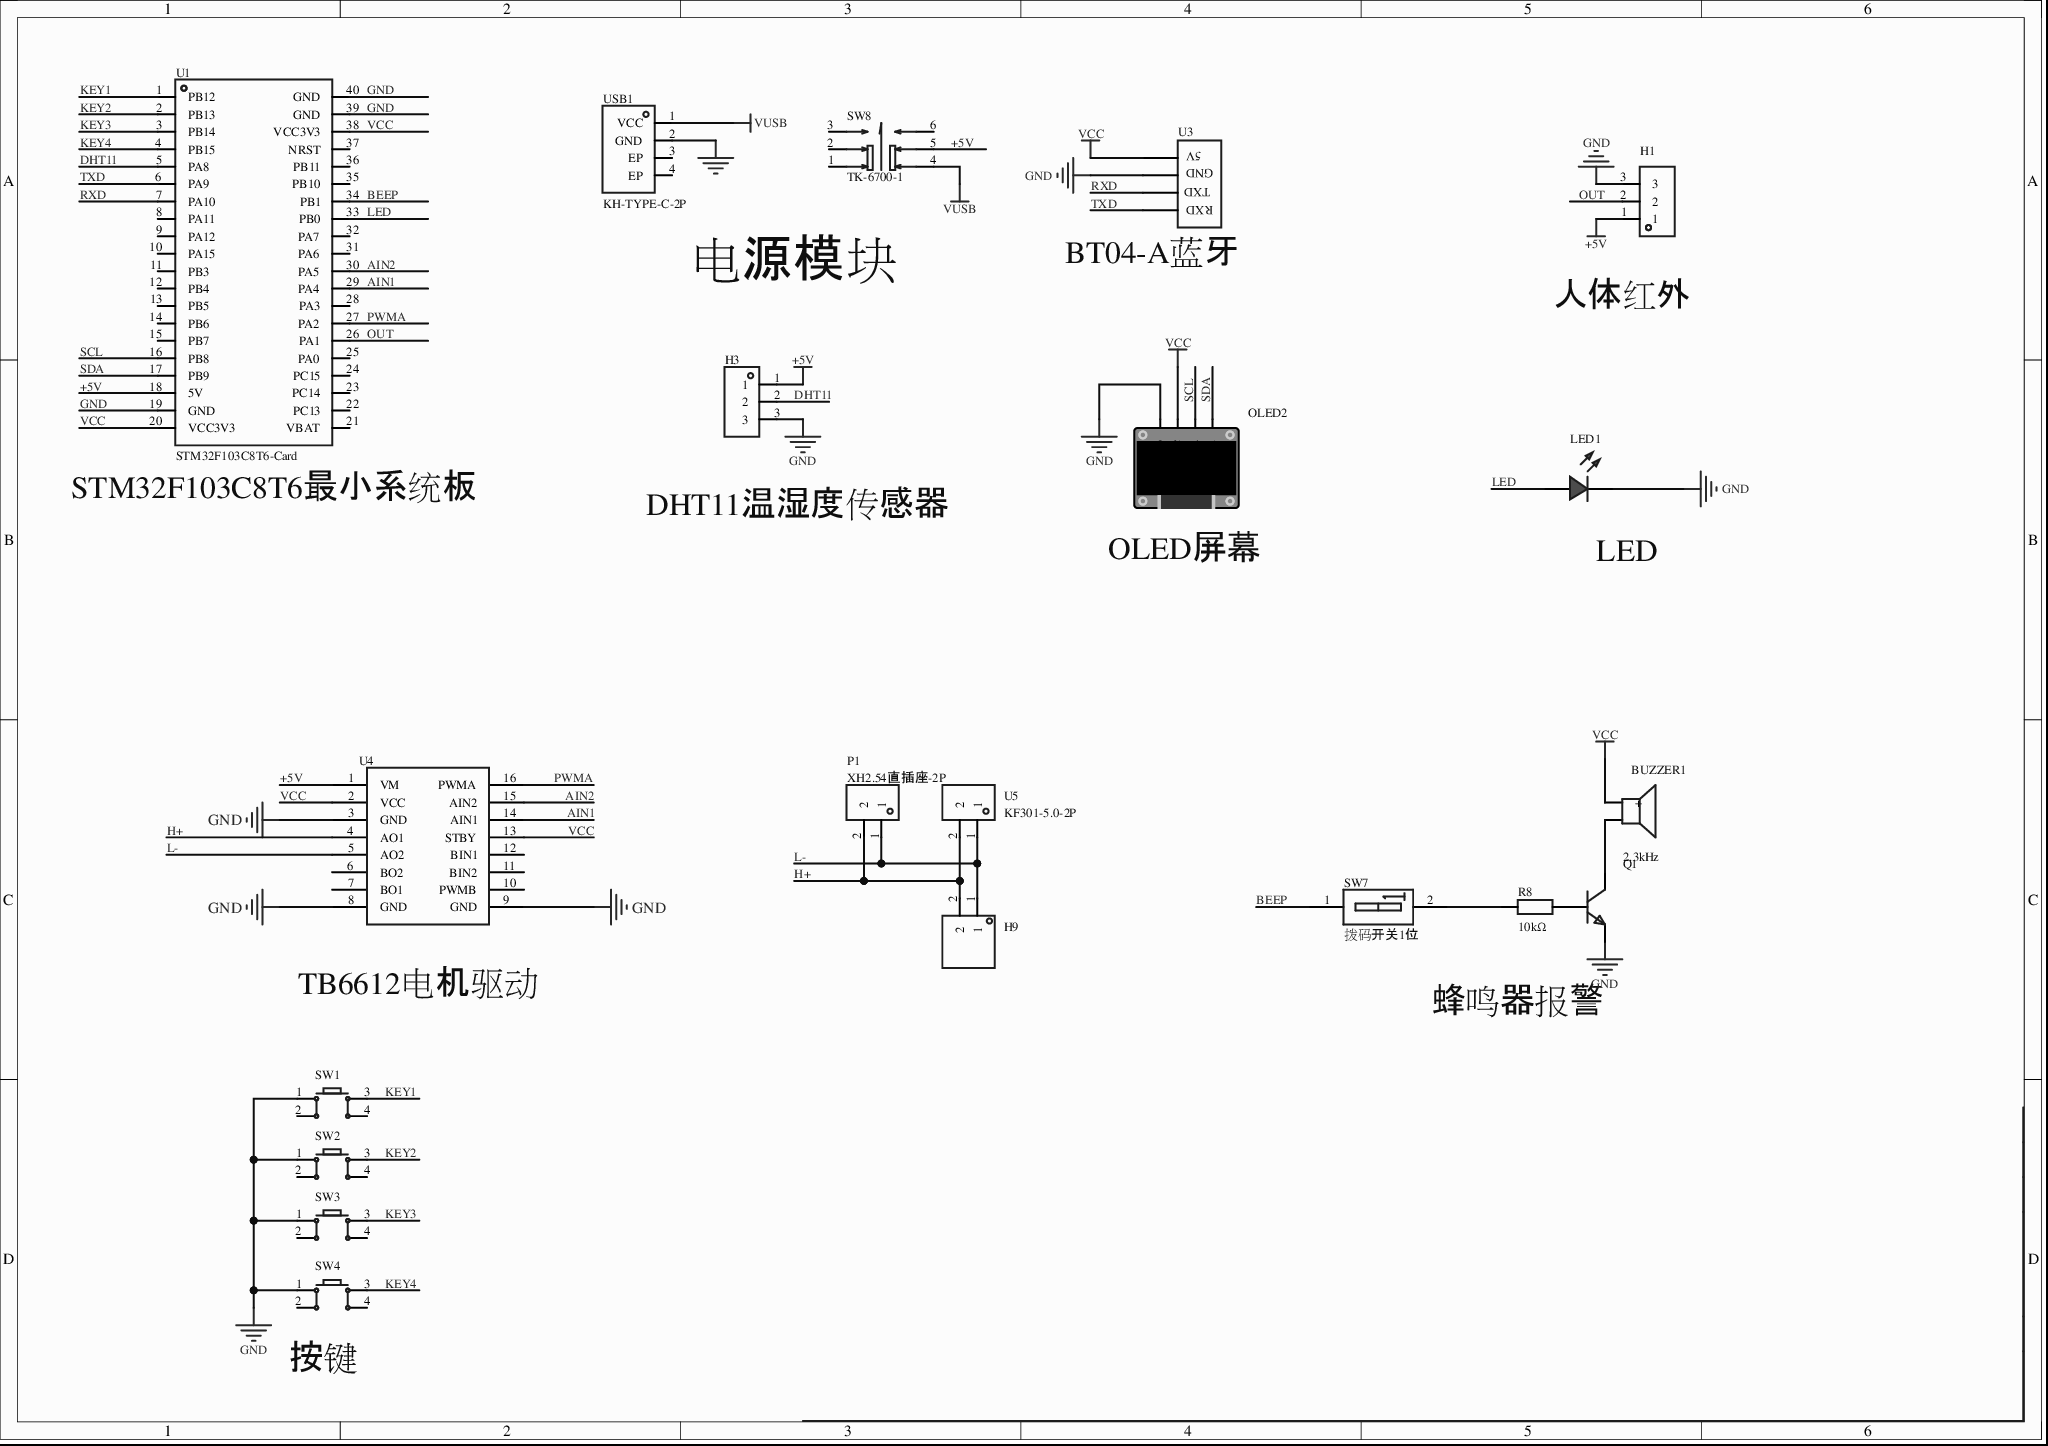
[diagram p0: MISC51405-3.schdoc]
# Altium project MISC51405-2.PrjPcb
1 sheet, 20 parts. Net scope: global (net labels, ports and power ports of the same name join across sheets).
Board file: MISC51405.pcbdoc

## Sheet MISC51405-3.schdoc
size 297 x 209 mm; Version: V1.0; @Project Name: MISC51405; @Page Count: 1; @Update Date: 2026-05-25; @Create Date: 2026-05-25; @Schematic Name: MISC51405; @Page No: 1; @Create Time: 23:22:16; @Update Time: 17:32:40; @Board Name: MISC51405

### Parts
BUZZER1  2.3kHz  [BUZ-TH_BD12.0-P7.60-D0.6-FD]
H1  (no value)  [HDR-TH_3P-P2.54-V-F]
H3  (no value)  [HDR-TH_3P-P2.54-V-F]
H9  (no value)  [HDR-TH_2P-P2.54-V-M-1]
LED1  (no value)  [LED_TH-3mm]
OLED2  (no value)  [0.96OLED_4P]
P1  XH2.54直插座-2P  [CONN-TH_XH2.54-2P]
Q1  (no value)  [S8050_TO_92]
R8  10kΩ  [Res_1/4W]
SW1  (no value)  [SW-TH_4P-L6.0-W6.0-P4.50-LS6.5]
SW2  (no value)  [SW-TH_4P-L6.0-W6.0-P4.50-LS6.5]
SW3  (no value)  [SW-TH_4P-L6.0-W6.0-P4.50-LS6.5]
SW4  (no value)  [SW-TH_4P-L6.0-W6.0-P4.50-LS6.5]
SW7  拨码开关1位  [SW-TH_2P-L3.9-W9.9-P2.54-LS7.6]
SW8  TK-6700-1  [SW-TH_TK-6700-1]
U1  STM32F103C8T6-Card  [CONN-TH_L53.3-W22.9_STM32F103C8T6-CARD]
U3  (no value)  [BT04-A]
U4  (no value)  [tb6612]
U5  KF301-5.0-2P  [CONN-TH_P5.00_KF301-5.0-2P]
USB1  KH-TYPE-C-2P  [USB-SMD_KH-TYPE-C-2P]

### Nets
+5V: H1.1 H3.1 SW8.5 U1.18(5V) U4.1(VM)
GND: H1.3 H3.3 LED1.2(A) OLED2.1(GND) Q1.1(E) SW1.1 SW2.1 SW3.1 SW4.1 U1.19(GND) U1.39(GND) U1.40(GND) U3.3 U4.3(GND) U4.8(GND) U4.9(GND) USB1.2(GND)
VCC: BUZZER1.1(+) OLED2.2(VCC) U1.20(VCC3V3) U1.38(VCC3V3) U3.4 U4.2(VCC) U4.13(STBY)
VUSB: SW8.4 USB1.1(VCC)
AIN1: U1.29(PA4) U4.14(AIN1)
AIN2: U1.30(PA5) U4.15(AIN2)
BEEP: SW7.1(A1) U1.34(PB1)
DHT11: H3.2 U1.5(PA8)
H+: H9.2 P1.2 U4.4(AO1) U5.2
KEY1: SW1.3 U1.1(PB12)
KEY2: SW2.3 U1.2(PB13)
KEY3: SW3.3 U1.3(PB14)
KEY4: SW4.3 U1.4(PB15)
L-: H9.1 P1.1 U4.5(AO2) U5.1
LED: LED1.1(C) U1.33(PB0)
OUT: H1.2 U1.26(PA1)
PWMA: U1.27(PA2) U4.16(PWMA)
RXD: U1.7(PA10) U3.2
SCL: OLED2.3(SCL) U1.16(PB8)
SDA: OLED2.4(SDA) U1.17(PB9)
TXD: U1.6(PA9) U3.1
NetBUZZER1_2: BUZZER1.2 Q1.3(C)
NetQ1_2: Q1.2(B) R8.2
NetR8_1: R8.1 SW7.2(A2)

Not connected (* = marked no-connect by the designer): SW1 2 4; SW2 2 4; SW3 2 4; SW4 2 4; SW8 1* 2* 3* 6*; U1 8(PA11) 9(PA12) 10(PA15) 11(PB3) 12(PB4) 13(PB5) 14(PB6) 15(PB7) 21(VBAT) 22(PC13) 23(PC14) 24(PC15) 25(PA0) 28(PA3) 31(PA6) 32(PA7) 35(PB10) 36(PB11) 37(NRST); U4 6(BO2) 7(BO1) 10(PWMB) 11(BIN2) 12(BIN1); USB1 3(EP) 4(EP)

### Notes on the sheet
- 电源模块
- (near U3) BT04-A蓝牙
- (near H1) 人体红外
- (near U1) STM32F103C8T6最小系统板
- DHT11温湿度传感器
- OLED屏幕
- (near LED1) LED
- TB6612电机驱动
- 蜂鸣器报警
- (near SW4) 按键

### Library data of the parts
BUZZER1 = TMB12A05_C96093: 驱动方式:有源(内含驱动线路);构造类型:电磁式;额定电压:5V;频率:2.3kHz;声压(SPL):85dB@5V,10cm;; Manufacturer: 华能; 3D Model: 16ab50e14c5b4f2c986c135bdba60e37; 3D Model Transform: 472.44,472.176,0,90,0,0,-0.787,0,-177.165; Technology Type: 电磁式; Rated Voltage: 5V; Operating Voltage: 4V~8V; AddInBom: yes; ModelName: BUZ-TH_D12.0-H9.5-P7.60; Symbol: TMB12A05; Device: TMB12A05_C96093; LCSC Part Name: TMB12A05; Supplier Part: C96093; Manufacturer Part: TMB12A05; Supplier Footprint: 插件,D=12mm; JLCPCB Part Class: Extended Part; Datasheet: https://atta.szlcsc.com/upload/public/pdf/source/20170522/1495448324811.pdf; Supplier: LCSC; Oscillator Circuit: 有源(内含驱动线路); Value: 2.3kHz; Sound Pressure Level (SPL): 85dB@5V,10cm; Diameter (φD): 12mm; Height: 9.8mm; ConvertToPcb: yes; FootprintName: BUZ-TH_BD12.0-P7.60-D0.6-FD
H1 = HDR-F_2.54_1x3P: Symbol: PM254V-11-03-H85; ConvertToPcb: yes; ModelId: f3b3cc5aae9641bf9e56fc160cef875b; ModelName: HDR2.54-F-LI-1X3P; ModelTransform: 299.9994,100,0,0,0,0,0,0,-118.11; Device: HDR-F_2.54_1x3P; FootprintName: HDR-TH_3P-P2.54-V-F; AddInBom: yes; SupplierPart: C541850; Supplier Footprint: 插件
H3 = HDR-F_2.54_1x3P: Symbol: PM254V-11-03-H85; 3D Model: f3b3cc5aae9641bf9e56fc160cef875b; 3D Model Transform: 299.9994,100,0,0,0,0,0,0,-118.11; ConvertToPcb: yes; ModelName: HDR2.54-F-LI-1X3P; Device: HDR-F_2.54_1x3P; Supplier Part: C541850; Supplier Footprint: 插件; FootprintName: HDR-TH_3P-P2.54-V-F; AddInBom: yes
H9 = HDR-M_2.54_1x2P: Symbol: 210S-1*2P L=11.6MMGold-plated black; ConvertToPcb: yes; ModelId: 79b2e9f2d70a4d68a1b7098f27c6d4c50819f05c4eef4c71ace90d822a990e87; ModelName: HDR-M-2.54_1x2; ModelTransform: 200,100,0,0,0,0,0,0,-118.11; Device: HDR-M_2.54_1x2P; AddInBom: yes; SupplierPart: C124375; Supplier Footprint: 插件; FootprintName: HDR-TH_2P-P2.54-V-M-1
LED1 = LED_TH-R_3mm: ConvertToPcb: yes; ModelId: a497c992633541038a38947cdc58012f0819f05c4eef4c71ace90d822a990e87; ModelName: LED-TH-3mm_R; ModelTransform: 141.274,153.327,0,0,0,0,-5.984,0,-137.795; Symbol: LED_TH-R; Device: LED_TH-R_3mm; AddInBom: yes; FootprintName: LED_TH-3mm; Supplier Footprint: 插件
OLED2 = 0.96OLED模块_4P: ConvertToPcb: yes; ModelId: 79c000fdb68d45a296c2e9bedf4f9055; ModelTransform: 1393.69792,1318.895,0,0,0,0,0,-560.079,-137.795; Symbol: 0.96OLED模块_4P; Device: 0.96OLED模块_4P; AddInBom: yes; FootprintName: 0.96OLED_4P; Supplier Footprint: 插件; ModelName: 0.96OLED_4P
P1 = XH2.54直插座-2P: AddInBom: yes; ModelId: c3cc11bd8b8748c1ae6bc231aac3a1ff0819f05c4eef4c71ace90d822a990e87; ModelTransform: 296.889,230.315,0,0,0,0,0,26.653,-137.795; Symbol: XH2.54直插座-2P; Device: XH2.54直插座-2P; LCSC Part Name: XH2.54直插座-2P; SupplierPart: C9900016957; ManufacturerPart: XH2.54直插座-2P; Supplier Footprint: XH2.54-2; JLCPCB Part Class: Extended Part; Supplier: LCSC; ConvertToPcb: yes; FootprintName: CONN-TH_XH2.54-2P; ModelName: CONN-TH_XH2.54-2P
Q1 = S8050_TO_NPN: 3D Model: aafe8e06f2154e7c93506efd0d6632dd; 3D Model Transform: 180.78,141.44,417.3,0,0,0,0,0,-200; ConvertToPcb: yes; ModelName: TO-92-3_L4.9-W3.7-P1.27-L; Symbol: S8050_TO_NPN; Device: S8050_TO_NPN; Supplier Footprint: TO-92; AddInBom: yes; FootprintName: S8050_TO_92
R8 = Res_AXIAL-1/4W: Symbol: 电阻; 3D Model: 463263665006444ab7a47bd11b0cf956; 3D Model Transform: 427.165,94.32816,0,0,0,0,0,0,-196.85; AddInBom: yes; ModelName: RES-TH_BD2.4-L6.3-P10.30-D0.6; Device: Res_AXIAL-1/4W; Value: 10kΩ; Supplier Footprint: 轴向引线; ConvertToPcb: yes; FootprintName: Res_1/4W
SW1-SW4 = Key_TH_6x6x6: 触点电流:50mA;额定电压(DC):12V;绝缘电阻:100MΩ;电路结构:单刀单掷;安装方式:直插;按钮形状:圆形按钮;按钮/盖帽颜色:黑色;作用力:260gf@±30gf;工作温度:-25℃~+70℃;引脚样式:PC引脚;开关长度:6mm;开关宽度:6mm;开关高度:6mm;带支架:否;; Symbol: 轻触按键; AddInBom: yes; ModelId: 20eee248bc684ccd8cbdbb1d0d91ec6f0819f05c4eef4c71ace90d822a990e87; ModelName: SW-TH_4P-L6.0-W6.0-H5.0-LS6.5-P4.50; ModelTransform: 236.22,323.03,0,90,0,0,0,0,-137.795; Device: Key_TH_6x6x6; FootprintName: SW-TH_4P-L6.0-W6.0-P4.50-LS6.5; ConvertToPcb: yes; Supplier Footprint: 插件
SW7 = NDS-01V_C501305: 正拨高杆; 3D Model: a6fe51954c31461ebc9e88beb6e51f3d0819f05c4eef4c71ace90d822a990e87; 3D Model Transform: 161.417,389.763,0,270,0,0,0,0,-125.984; AddInBom: yes; ModelName: SW-TH_L4.0-W9.9-H5.4-P2.54-B; Symbol: NDS-01V; Device: NDS-01V_C501305; LCSC Part Name: 拨码开关; Supplier Part: C501305; Manufacturer Part: 拨码开关1位; Supplier Footprint: DIP; JLCPCB Part Class: Extended Part; Supplier: LCSC; ConvertToPcb: yes; FootprintName: SW-TH_2P-L3.9-W9.9-P2.54-LS7.6
SW8 = TK-6700-1: Manufacturer: Yuandi(元迪); 3D Model: 1dccfbf2ceb24a728093c1f6ee61932a; 3D Model Transform: 275.59,275.59,0,90,0,0,0,0,-137.795; AddInBom: yes; Symbol: TK-6700-1; Device: TK-6700-1; LCSC Part Name: 自锁开关7*7*12.7有声有锁高导高柄插件双排6P按键开关带锁DIP六脚; Supplier Part: C528782; Manufacturer Part: TK-6700-1; Supplier Footprint: 插件; JLCPCB Part Class: Extended Part; Datasheet: https://atta.szlcsc.com/upload/public/pdf/source/20200831/C528782_58F076EBF84BD8A9E2DE38DB1C0986D4.pdf; Supplier: LCSC; ConvertToPcb: yes; FootprintName: SW-TH_TK-6700-1; ModelName: SW-TH_TK-6700-1
U1 = STM32F103C8T6-Card: AddInBom: yes; Device: STM32F103C8T6-Card; Symbol: STM32F103C8T6-CARD; FootprintName: CONN-TH_L53.3-W22.9_STM32F103C8T6-CARD; LCSC Part Name: STM32F103C8T6-Card; SupplierPart: C9900077949; ManufacturerPart: STM32F103C8T6-Card; Supplier Footprint: 插件; Supplier: LCSC; ConvertToPcb: yes
U3 = bt04: Symbol: bt04_2; AddInBom: yes; ModelId: eb640bf7e8924172bf5da6313bfb275c43cd9731070e40ef8f44b4d173fb7123; ModelTransform: 448.8179849815368,622.0460075092316,90.5509981226921,0,0,0,0,0,0; Device: bt04; ConvertToPcb: yes; ModelName: BT04; FootprintName: BT04-A
U4 = tb6612: AddInBom: yes; Symbol: tb6612; Device: tb6612; JLCPCB Part Class: 扩展库; ConvertToPcb: yes; FootprintName: tb6612
U5 = KF301-5.0-2P: 结构:1x2P;间距:5mm;颜色:蓝色;安装方式:直插;排数:1;每排PIN数:2;额定电流:17A;额定电压:250V;线规 - AWG:14~22;线规 - 平方毫米:1.5;工作温度:-30℃~+120℃;; Manufacturer: KEFA(科发); AddInBom: yes; ModelId: 442de893d0fc4728b9e5c7abc29ccda50819f05c4eef4c71ace90d822a990e87; ModelTransform: 417.322,299.21594,0,0,0,0,11.811,7.874,-137.795; Number of Positions or Pins: 1x2P; Pitch: 5mm; Number of PINs Per Row: 2; Current Rating: 17A; Voltage Rating (Max): 250V; Wire Gauge - AWG: 14~22; Wire Gauge - mm2: 1.5; Symbol: KF301-5.0-2P; Device: KF301-5.0-2P; LCSC Part Name: 1x2P 5mm 直插 排数:1 每排P数:2; SupplierPart: C474881; ManufacturerPart: KF301-5.0-2P; Supplier Footprint: 插件,P=5mm; JLCPCB Part Class: Extended Part; Datasheet: https://item.szlcsc.com/datasheet/KF301-5.0-2P/481499.html; Supplier: LCSC; ConvertToPcb: yes; FootprintName: CONN-TH_P5.00_KF301-5.0-2P; ModelName: CONN-TH_P5.00_KF301-5.0-2P; Color: 蓝色; Mounting Type: 直插; Number of Pins: 2P; Number of Rows: 1; Operating Temperature: -30℃~+120℃
USB1 = KH-TYPE-C-2P: 连接器类型:Type-C;标准:-;公母:-;端口数量:-;触点数量:2P;安装方式:-;额定电流 - 电源:-;触头材质:-;触头镀层:-;工作温度范围:-;; Manufacturer: kinghelm(金航标); 3D Model: 4464b34a7d0f48c2b8c2350e914c93f5; 3D Model Transform: 352.362,255.31449,0,0,0,0,0,-49.213,-98.425; Connector Type: Type-C; Number of Contacts: 2P; Current Rating-Power: 3A; Voltage Rating: 20V; Connect-Disconnect Life: 5千次; AddInBom: yes; Symbol: KH-TYPE-C-2P; Device: KH-TYPE-C-2P; LCSC Part Name: Type-C; Supplier Part: C2919656; Manufacturer Part: KH-TYPE-C-2P; Supplier Footprint: 插件; JLCPCB Part Class: Extended Part; Datasheet: https://atta.szlcsc.com/upload/public/pdf/source/20220707/620587A9E0589B27D96D3CEE595CBC98.pdf; Supplier: LCSC; Standard: -; Gender: -; Number of Ports: -; Mounting Style: -; Current Rating - Power (Max): -; Contact Material: -; Contact Plating: -; Operating Temperature Range: -; Protocol Standard: -; Mounting Type: 弯插; Length: 6.43mm; Operating Temperature: -25℃~+85℃; ConvertToPcb: yes; FootprintName: USB-SMD_KH-TYPE-C-2P; ModelName: USB-SMD_KH-TYPE-C-2P